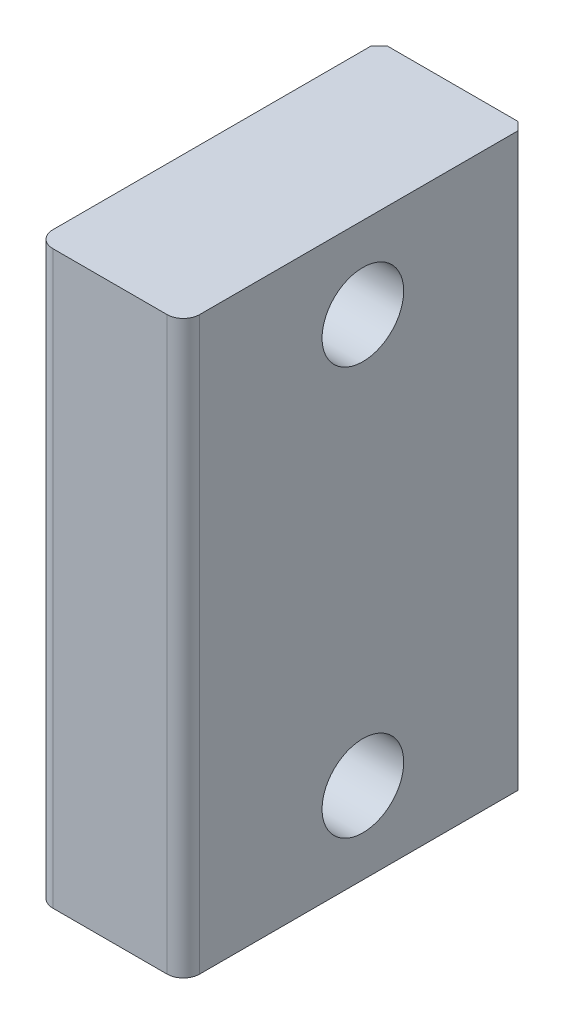
from build123d import *

# Parameters (mm, degrees)
SKETCH1_W             = 9
SKETCH1_H             = 35
BOSS_EXTRUDE1_DEPTH   = 21
M6_TAPPED_HOLE1_D     = 5
M6_TAPPED_HOLE1_DEPTH = 15
M6_TAPPED_HOLE1_TIP   = 1.502151548
M4_TAPPED_HOLE1_D     = 3.3
M4_TAPPED_HOLE1_DEPTH = 15
M4_TAPPED_HOLE1_TIP   = 0.991420021
FILLET1_R             = 1
CHAMFER1_SIZE         = 0.5


with BuildPart() as part:
    # Sketch1 → Boss-Extrude1 (new body)
    with BuildSketch(Plane.XY):
        with Locations((4.5, 0)):
            Rectangle(SKETCH1_W, SKETCH1_H)
    extrude(amount=BOSS_EXTRUDE1_DEPTH)

    # M6 Tapped Hole1
    with Locations(Plane(origin=(9, 0, 0), x_dir=(0, 0, -1), z_dir=(1, 0, 0))):
        with Locations((-10, 12.5), (-10, -12.5)):
            Hole(M6_TAPPED_HOLE1_D / 2, depth=M6_TAPPED_HOLE1_DEPTH)
            with Locations((0, 0, -(M6_TAPPED_HOLE1_DEPTH + M6_TAPPED_HOLE1_TIP / 2))):  # 118° drill point
                Cone(0, M6_TAPPED_HOLE1_D / 2, M6_TAPPED_HOLE1_TIP, mode=Mode.SUBTRACT)

    # M4 Tapped Hole1
    with Locations(Plane(origin=(0, 0, 0), x_dir=(-1, 0, 0), z_dir=(0, 0, -1))):
        with Locations((-4.5, 4.5), (-4.5, -4.5)):
            Hole(M4_TAPPED_HOLE1_D / 2, depth=M4_TAPPED_HOLE1_DEPTH)
            with Locations((0, 0, -(M4_TAPPED_HOLE1_DEPTH + M4_TAPPED_HOLE1_TIP / 2))):  # 118° drill point
                Cone(0, M4_TAPPED_HOLE1_D / 2, M4_TAPPED_HOLE1_TIP, mode=Mode.SUBTRACT)

    # Fillet1
    fillet1_edges = [part.edges().sort_by_distance(p)[0] for p in [
        (9, 0, 21),
        (0, 0, 21),
    ]]
    fillet(fillet1_edges, radius=FILLET1_R)

    # Chamfer1
    chamfer1_edges = [part.edges().sort_by_distance(p)[0] for p in [
        (9, 0, 0),
        (0, 0, 0),
    ]]
    chamfer(chamfer1_edges, length=CHAMFER1_SIZE)


solid = part.part
